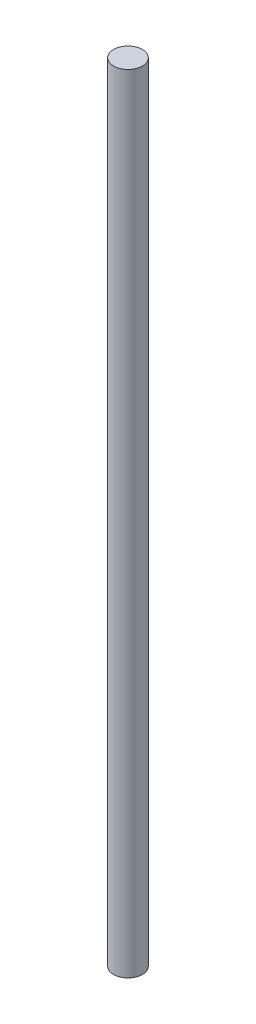
from build123d import *

# Parameters (mm, degrees)
SKETCH1_R           = 1.5
BOSS_EXTRUDE1_DEPTH = 82


with BuildPart() as part:
    # Sketch1 → Boss-Extrude1 (new body)
    with BuildSketch(Plane(origin=(0, 0, 0), x_dir=(1, 0, 0), z_dir=(0, 1, 0))):
        with Locations(Location((0, 0, 0), (0, 0, 270))):
            Circle(SKETCH1_R)
    extrude(amount=BOSS_EXTRUDE1_DEPTH)


solid = part.part
